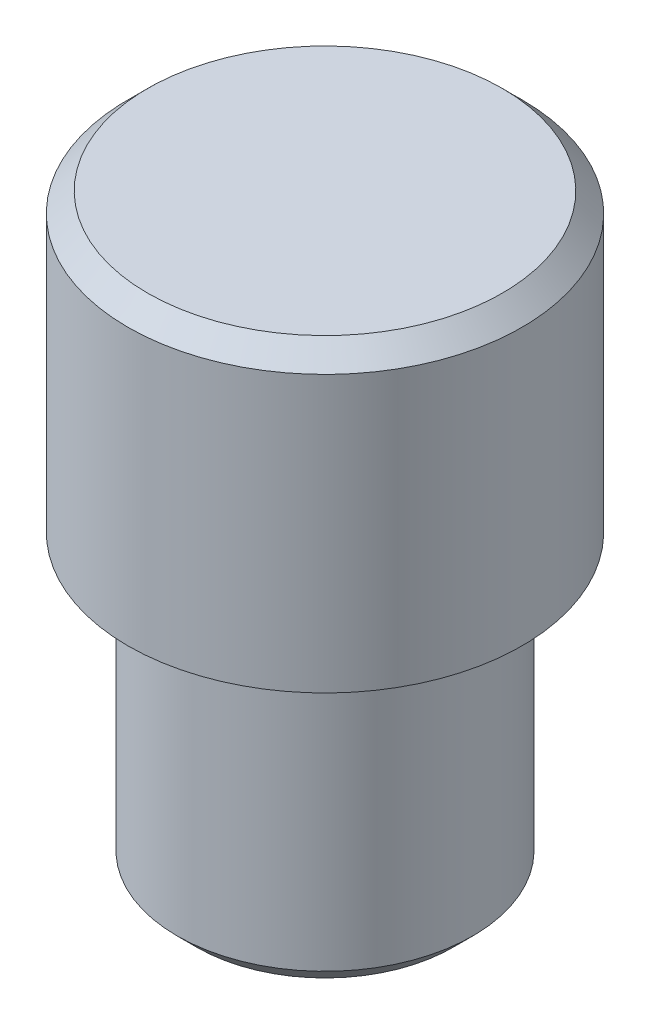
SolidWorks part; units mm, degrees
material "6061 合金"
ref_plane "Front Plane" through (0, 0, 0) normal (0, 0, 1) x (1, 0, 0)
ref_plane "Top Plane" through (0, 0, 0) normal (0, 1, 0) x (1, 0, 0)
ref_plane "Right Plane" through (0, 0, 0) normal (1, 0, 0) x (0, 0, -1)
sketch "Sketch1" plane through (0, 0, 0) normal (0, 1, 0) x (1, 0, 0)
  circle A0 centre (0, 0) radius 1.5
  dimension "D1" = 3
extrude "Boss-Extrude1" add sketch "Sketch1" along normal blind 3
sketch "Sketch2" plane through (0, 3, 0) normal (0, 1, 0) x (1, 0, 0)
  circle A0 centre (0, 0) radius 2
  dimension "D1" = 4
extrude "Boss-Extrude2" add sketch "Sketch2" along normal blind 3
chamfer "Chamfer1" distance 0.2 angle 45 2 edges at (0, 0, 1.5) (0, 6, 2)
